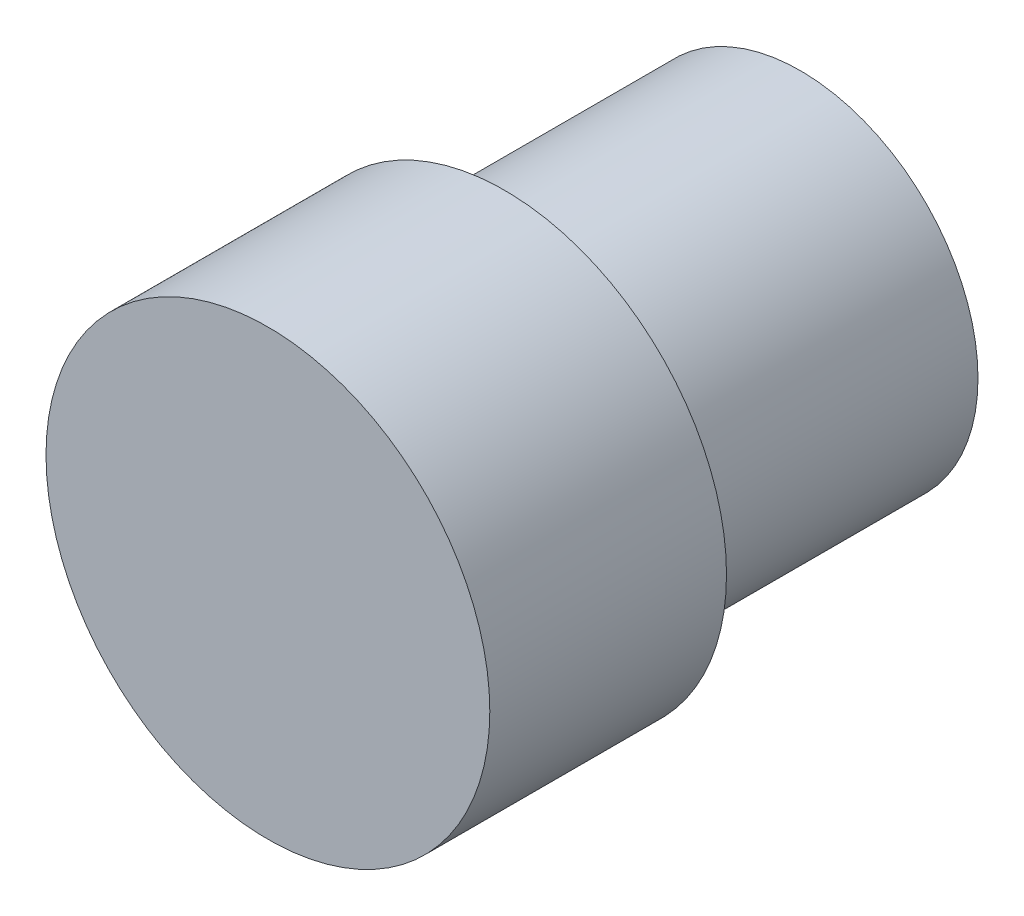
SolidWorks part; units mm, degrees
ref_plane "前视基准面" through (0, 0, 0) normal (0, 0, 1) x (1, 0, 0)
ref_plane "上视基准面" through (0, 0, 0) normal (0, 1, 0) x (1, 0, 0)
ref_plane "右视基准面" through (0, 0, 0) normal (1, 0, 0) x (0, 0, -1)
other "Configuration Table"
sketch "草图1" plane through (0, 0, 0) normal (0, 0, 1) x (1, 0, 0)
  circle A0 centre (0, 0) radius 6
  point P0 (0, 0)
  dimension "D1" = 12
extrude "凸台-拉伸1" add sketch "草图1" against normal blind 10
sketch "草图2" plane through (0, 0, 0) normal (0, 0, 1) x (1, 0, 0)
  circle A0 centre (0, 0) radius 7.5
  point P0 (0, 0)
  dimension "D1" = 15
extrude "凸台-拉伸2" add sketch "草图2" along normal blind 8
